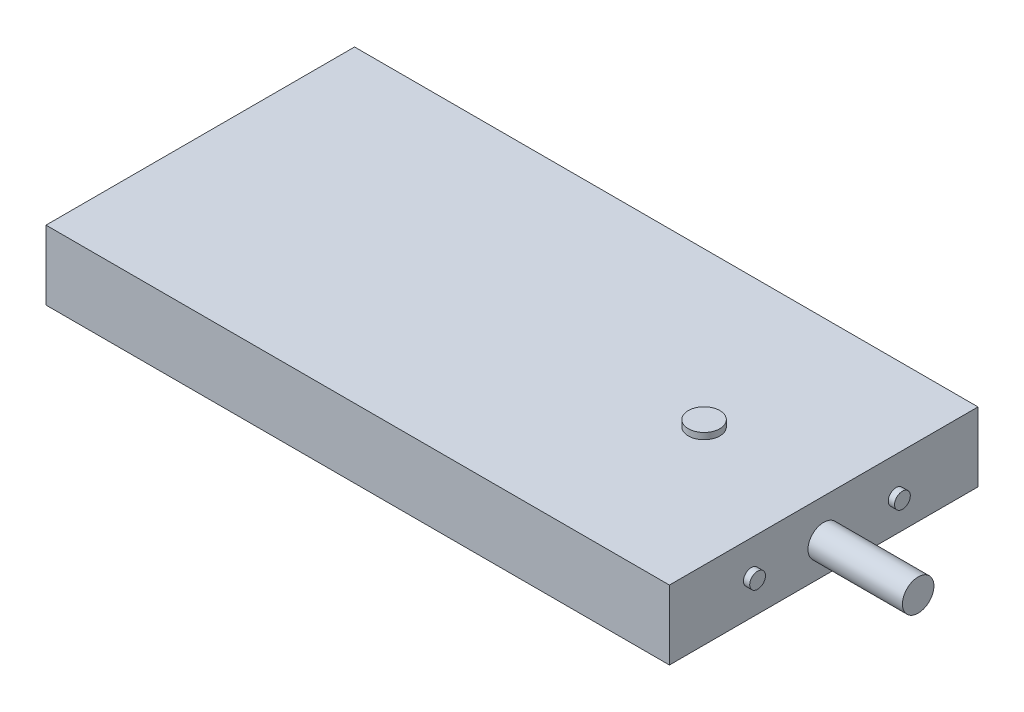
SolidWorks part; units mm, degrees
ref_plane "Front Plane" through (0, 0, 0) normal (0, 0, 1) x (1, 0, 0)
ref_plane "Top Plane" through (0, 0, 0) normal (0, 1, 0) x (1, 0, 0)
ref_plane "Right Plane" through (0, 0, 0) normal (1, 0, 0) x (0, 0, -1)
sketch "Sketch1" plane through (0, 0, 0) normal (0, 1, 0) x (1, 0, 0)
  line L1 (-99, -49) -> (99, -49)
  line L2 (-99, -49) -> (-99, 49)
  line L3 (-99, 49) -> (99, 49)
  line L4 (99, -49) -> (99, 49)
  line L5 (-99, -49) -> (99, 49) construction
  line L6 (-99, 49) -> (99, -49) construction
  point P0 (0, 0)
  dimension "D1" = 198
  dimension "D2" = 98
extrude "Boss-Extrude1" add sketch "Sketch1" along normal blind 22
sketch "Sketch2" plane through (99, 0, 0) normal (1, 0, 0) x (0, 0, -1)
  circle A0 centre (0, 9.76) radius 5
  dimension "D1" = 10
extrude "Boss-Extrude2" add sketch "Sketch2" along normal blind 30
sketch "Sketch3" plane through (0, 22, 0) normal (0, 1, 0) x (1, 0, 0)
  line L0 (99, -49) -> (99, 49) construction
  circle A0 centre (61, 0) radius 5
  dimension "D1" = 10
  dimension "D2" = 38
extrude "Boss-Extrude3" add sketch "Sketch3" along normal blind 2
sketch "Sketch4" plane through (99, 0, 0) normal (1, 0, 0) x (0, 0, -1)
  line L0 (49, 22) -> (49, 0) construction
  line L1 (-49, 22) -> (-49, 0) construction
  circle A0 centre (23, 10.3308) radius 2.5
  circle A1 centre (-23, 11.3252) radius 2.5
  dimension "D1" = 5
  dimension "D2" = 5
  dimension "D3" = 26
  dimension "D4" = 26
extrude "Boss-Extrude4" add sketch "Sketch4" along normal blind 2
